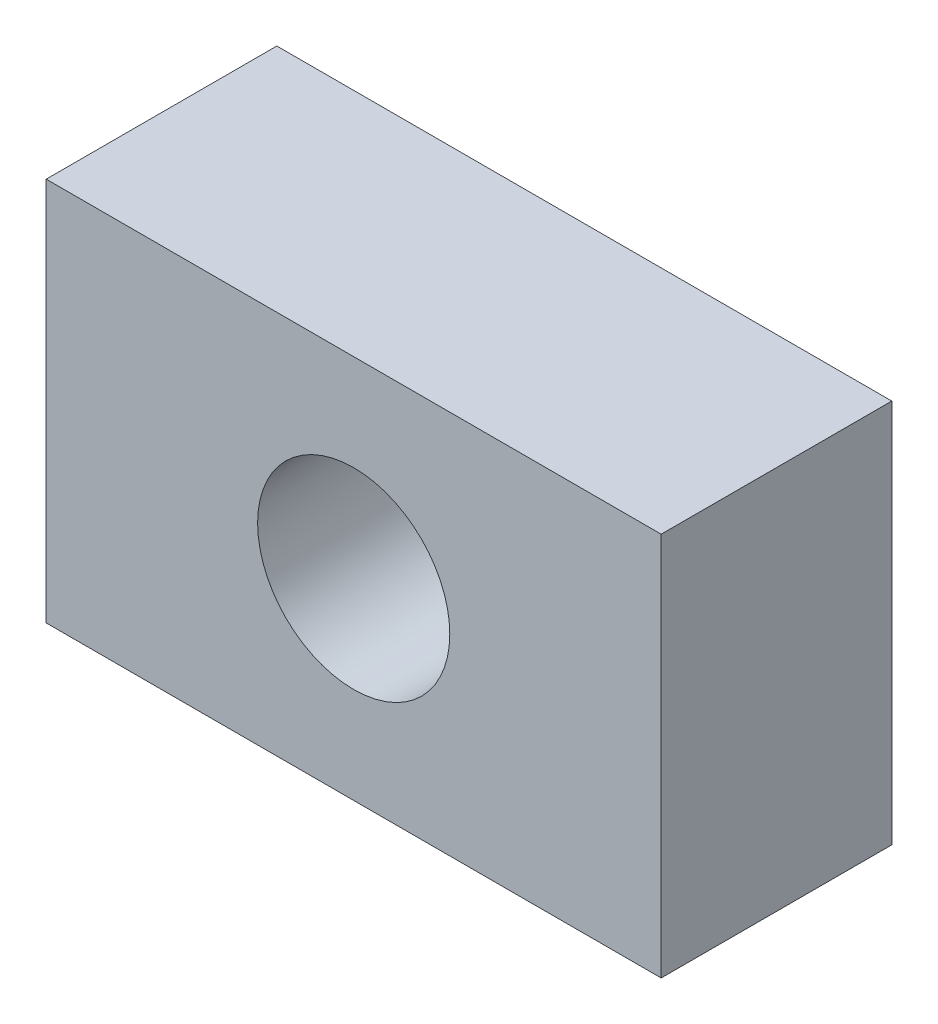
from build123d import *

# Parameters (mm, degrees)
SKETCH1_W           = 16
SKETCH1_H           = 10
BOSS_EXTRUDE1_DEPTH = 6
M6_TAPPED_HOLE1_D   = 5


with BuildPart() as part:
    # Sketch1 → Boss-Extrude1 (new body)
    with BuildSketch(Plane.XY):
        Rectangle(SKETCH1_W, SKETCH1_H)
    extrude(amount=BOSS_EXTRUDE1_DEPTH)

    # M6 Tapped Hole1 (through all)
    with Locations(Plane.XY.offset(6)):
        with Locations((0, 0)):
            Hole(M6_TAPPED_HOLE1_D / 2)


solid = part.part
